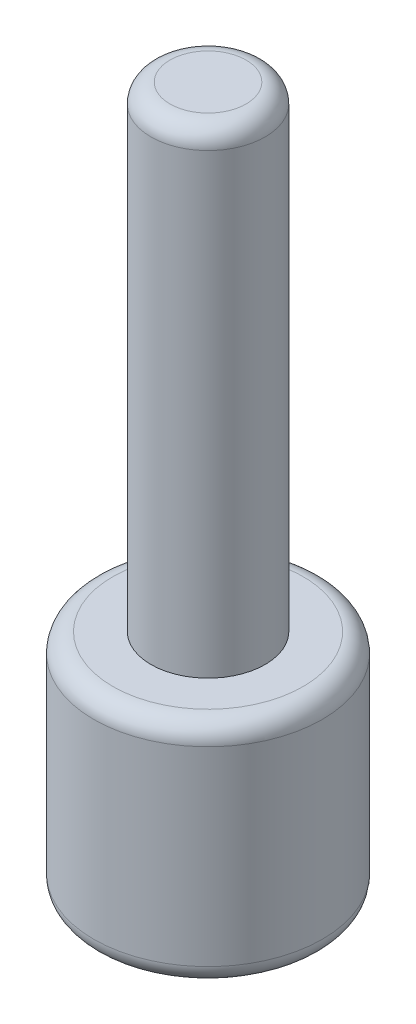
from build123d import *

# Parameters (mm, degrees)
SKETCH_1_R      = 6
EXTRUDE_1_DEPTH = 12
SKETCH_2_R      = 3
EXTRUDE_2_DEPTH = 25
FILLET_1_R      = 1


with BuildPart() as part:
    # 草图1 → 凸台-拉伸1 (new body)
    with BuildSketch(Plane(origin=(0, 0, 0), x_dir=(1, 0, 0), z_dir=(0, 1, 0))):
        with Locations(Location((0, 0, 0), (0, 0, 270))):
            Circle(SKETCH_1_R)
    extrude(amount=EXTRUDE_1_DEPTH)

    # 草图2 → 凸台-拉伸2 (add)
    with BuildSketch(Plane(origin=(0, 12, 0), x_dir=(1, 0, 0), z_dir=(0, 1, 0))):
        with Locations(Location((0, 0, 0), (0, 0, 270))):
            Circle(SKETCH_2_R)
    extrude(amount=EXTRUDE_2_DEPTH)

    # 圆角1
    fillet_1_edges = [part.edges().sort_by_distance(p)[0] for p in [
        (0, 0, -6),
        (0, 12, -6),
        (0, 37, -3),
    ]]
    fillet(fillet_1_edges, radius=FILLET_1_R)


solid = part.part
